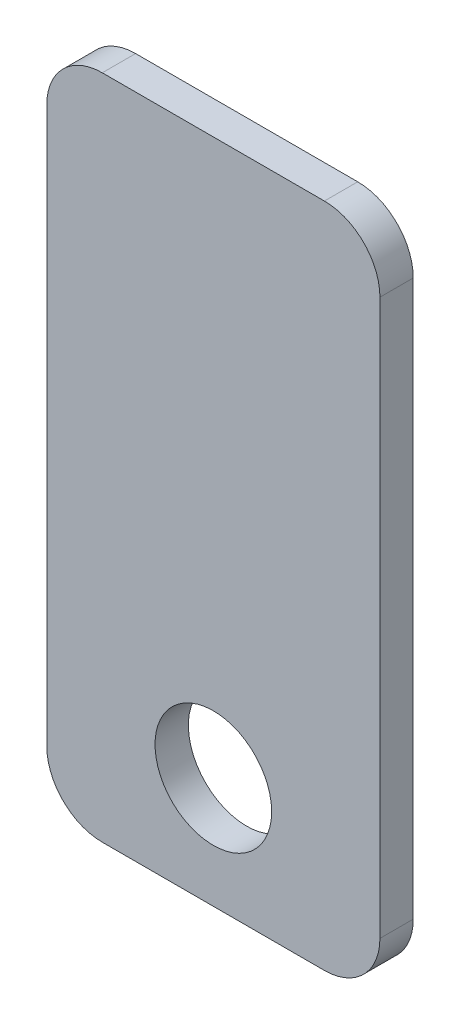
from build123d import *

# Parameters (mm, degrees)
SKETCH1_R           = 5.25
BOSS_EXTRUDE1_DEPTH = 3


with BuildPart() as part:
    # Sketch1 → Boss-Extrude1 (new body)
    with BuildSketch(Plane.XY):
        with BuildLine():
            Line((-10, 30), (10, 30))
            ThreePointArc((10, 30), (13.535533906, 28.535533906), (15, 25))
            Line((15, 25), (15, -25))
            ThreePointArc((15, -25), (13.535533906, -28.535533906), (10, -30))
            Line((10, -30), (-10, -30))
            ThreePointArc((-10, -30), (-13.535533906, -28.535533906), (-15, -25))
            Line((-15, -25), (-15, 25))
            ThreePointArc((-15, 25), (-13.535533906, 28.535533906), (-10, 30))
        make_face()
        with Locations((0, -20)):
            Circle(SKETCH1_R, mode=Mode.SUBTRACT)
    extrude(amount=BOSS_EXTRUDE1_DEPTH)


solid = part.part
